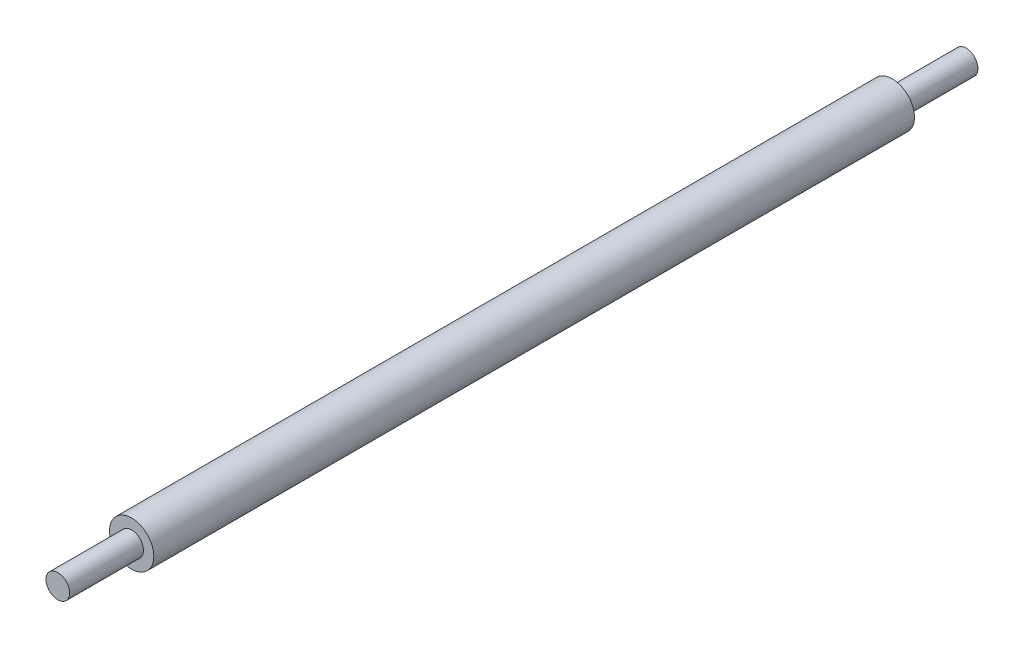
SolidWorks part; units mm, degrees
material "K"
ref_plane "Front" through (0, 0, 0) normal (0, 0, 1) x (1, 0, 0)
ref_plane "Top" through (0, 0, 0) normal (0, 1, 0) x (1, 0, 0)
ref_plane "Right" through (0, 0, 0) normal (1, 0, 0) x (0, 0, -1)
sketch "Sketch1" plane through (0, 0, 0) normal (0, 0, 1) x (1, 0, 0)
  circle A0 centre (0, 0) radius 15
  dimension "D1" = 30
extrude "Boss-Extrude1" add sketch "Sketch1" along normal mid plane 515
sketch "Sketch2" plane through (0, 0, 257.5) normal (0, 0, 1) x (1, 0, 0)
  circle A0 centre (0, 0) radius 8
  dimension "D1" = 16
extrude "Boss-Extrude2" add sketch "Sketch2" along normal blind 50
cosmetic thread "Cosmetic Thread2" parameters "D2"=13.835
sketch "Sketch3" plane through (0, 0, -257.5) normal (0, 0, -1) x (-1, 0, 0)
  circle A0 centre (0, 0) radius 8
  dimension "D1" = 16
extrude "Boss-Extrude3" add sketch "Sketch3" along normal blind 50
cosmetic thread "Cosmetic Thread1" parameters "D2"=13.835
equation "\"零件重量\"= IIF ( \"SW-质量\" > 100 , int ( \"SW-质量\" ) , \"SW-质量\" )"
